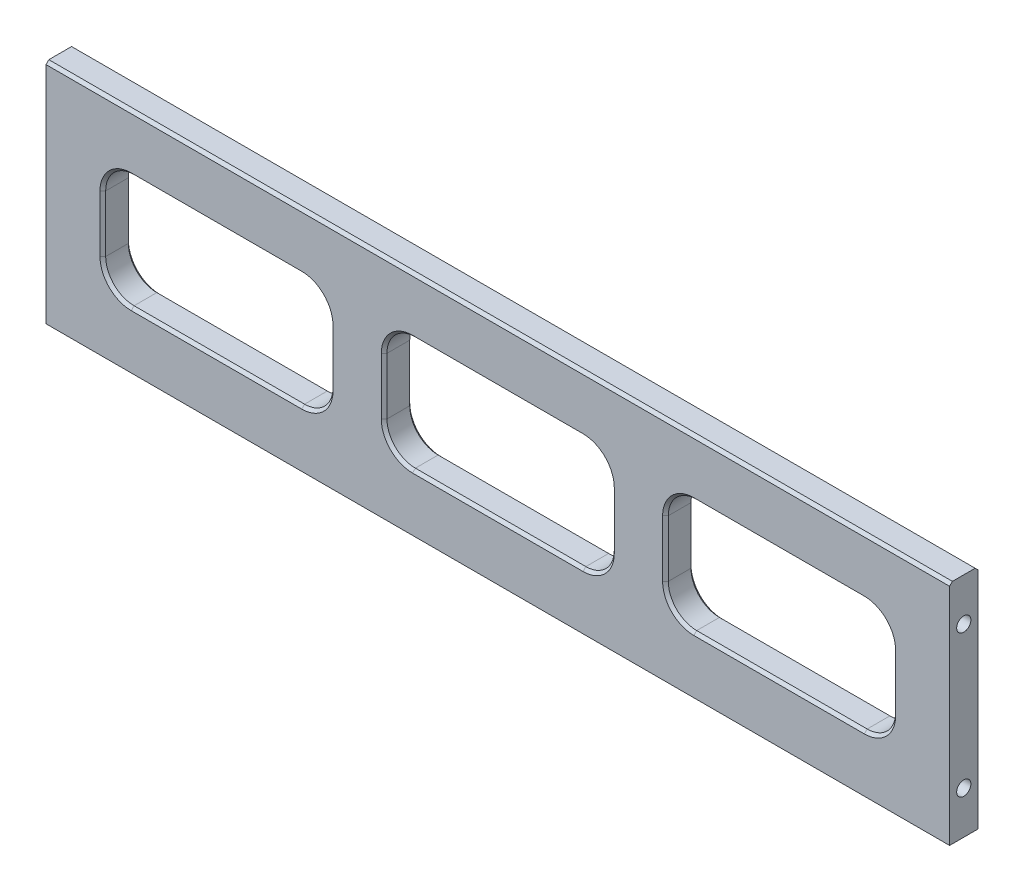
SolidWorks part; units mm, degrees
ref_plane "前视基准面" through (0, 0, 0) normal (0, 0, 1) x (1, 0, 0)
ref_plane "上视基准面" through (0, 0, 0) normal (0, 1, 0) x (1, 0, 0)
ref_plane "右视基准面" through (0, 0, 0) normal (1, 0, 0) x (0, 0, -1)
ref_plane "基准面4" through (0, 0, 10) normal (0, 0, 1) x (1, 0, 0)
sketch "草图1" plane through (0, 0, 10) normal (0, 0, 1) x (1, 0, 0)
  line L0 (-159, -20) -> (-159, -100)
  line L1 (-159, -100) -> (159, -100)
  line L2 (159, -100) -> (159, -20)
  line L3 (159, -20) -> (-159, -20)
extrude "凸台-拉伸1" add sketch "草图1" against normal blind 10
sketch "草图2" plane through (0, 0, 10) normal (0, 0, 1) x (1, 0, 0)
  line L0 (40, -80) -> (40, -40)
  line L1 (40, -40) -> (-40, -40)
  line L2 (-40, -40) -> (-40, -80)
  line L3 (-40, -80) -> (40, -80)
extrude "切除-拉伸1" cut sketch "草图2" against normal through all
sketch "草图3" plane through (0, 0, 10) normal (0, 0, 1) x (1, 0, 0)
  line L0 (139, -80) -> (139, -40)
  line L1 (139, -40) -> (59, -40)
  line L2 (59, -40) -> (59, -80)
  line L3 (59, -80) -> (139, -80)
extrude "切除-拉伸2" cut sketch "草图3" against normal through all
sketch "草图4" plane through (0, 0, 0) normal (0, 0, -1) x (-1, 0, 0)
  line L0 (59, -40) -> (59, -80)
  line L1 (59, -80) -> (139, -80)
  line L2 (139, -80) -> (139, -40)
  line L3 (139, -40) -> (59, -40)
extrude "切除-拉伸3" cut sketch "草图4" against normal through all
hole_wizard "Ø5.0 (5) 直径孔1" positions "草图6" profile "草图5" hole size "Ø5.0" standard "ANSI Metric"
sketch "草图6" plane through (-159, 0, 0) normal (-1, 0, 0) x (0, 0, 1)
  point P0 (5, -35)
  point P1 (5, -85)
sketch "草图5" plane through (-159, -35, 5) normal (0, 1, 0) x (0, 0, 1)
  line L0 (0, 0) -> (0, 16.5022)
  line L1 (0, 16.5022) -> (2.5, 15)
  line L2 (2.5, 15) -> (2.5, 0)
  line L5 (2.5, 0) -> (0, 0)
  line L10 (0, 16.5022) -> (-2.5, 15) construction
  line L11 (0, -6.35) -> (0, 107.95) construction
  dimension "孔直径" = 5
  dimension "孔深度" = 15
  dimension "导头角度" = 118
hole_wizard "Ø5.0 (5) 直径孔2" positions "草图8" profile "草图7" hole size "Ø5.0" standard "ANSI Metric"
sketch "草图8" plane through (159, 0, 0) normal (1, 0, 0) x (0, 0, -1)
  point P0 (-5, -35)
  point P1 (-5, -85)
sketch "草图7" plane through (159, -35, 5) normal (0, 1, 0) x (0, 0, -1)
  line L0 (0, 0) -> (0, 16.5022)
  line L1 (0, 16.5022) -> (2.5, 15)
  line L2 (2.5, 15) -> (2.5, 0)
  line L5 (2.5, 0) -> (0, 0)
  line L10 (0, 16.5022) -> (-2.5, 15) construction
  line L11 (0, -6.35) -> (0, 107.95) construction
  dimension "孔直径" = 5
  dimension "孔深度" = 15
  dimension "导头角度" = 118
hole_wizard "Ø5.0 (5) 直径孔3" positions "草图10" profile "草图9" hole size "Ø5.0" standard "ANSI Metric"
sketch "草图10" plane through (0, -100, 0) normal (0, -1, 0) x (-1, 0, 0)
  point P0 (121.5, -5)
  point P1 (40.5, -5)
  point P2 (-40.5, -5)
  point P3 (-121.5, -5)
sketch "草图9" plane through (-121.5, -100, 5) normal (1, 0, 0) x (0, 0, -1)
  line L0 (0, 0) -> (0, 16.5022)
  line L1 (0, 16.5022) -> (2.5, 15)
  line L2 (2.5, 15) -> (2.5, 0)
  line L5 (2.5, 0) -> (0, 0)
  line L10 (0, 16.5022) -> (-2.5, 15) construction
  line L11 (0, -6.35) -> (0, 107.95) construction
  dimension "孔直径" = 5
  dimension "孔深度" = 15
  dimension "导头角度" = 118
fillet "圆角1" radius 10 12 edges at (40, -40, 5) (139, -40, 5) (-40, -80, 5) (139, -80, 5) (-139, -40, 5) (59, -40, 5) (40, -80, 5) (-59, -40, 5) (-40, -40, 5) (-59, -80, 5) (-139, -80, 5) (59, -80, 5)
chamfer "倒角1" distance 1 angle 45 50 edges at (59, -60, 0) (61.9289, -42.9289, 0) (61.9289, -77.0711, 0) (99, -40, 0) (99, -80, 0) (136.0711, -42.9289, 0) (136.0711, -77.0711, 0) (139, -60, 0) (37.0711, -42.9289, 10) (0, -40, 10) (40, -60, 10) (-37.0711, -42.9289, 10) (37.0711, -77.0711, 10) (-40, -60, 10) (0, -80, 10) (-37.0711, -77.0711, 10) (136.0711, -42.9289, 10) (99, -40, 10) (139, -60, 10) (61.9289, -42.9289, 10) (136.0711, -77.0711, 10) (59, -60, 10) (99, -80, 10) (61.9289, -77.0711, 10) (40, -60, 0) (37.0711, -77.0711, 0) (37.0711, -42.9289, 0) (0, -80, 0) (0, -40, 0) (-37.0711, -77.0711, 0) (-37.0711, -42.9289, 0) (-40, -60, 0) (-136.0711, -42.9289, 10) (-99, -40, 10) (-139, -60, 10) (-61.9289, -42.9289, 10) (-136.0711, -77.0711, 10) (-59, -60, 10) (-99, -80, 10) (-61.9289, -77.0711, 10) (0, -20, 0) (0, -20, 10) (-99, -80, 0) (-61.9289, -77.0711, 0) (-136.0711, -77.0711, 0) (-59, -60, 0) (-139, -60, 0) (-61.9289, -42.9289, 0) (-136.0711, -42.9289, 0) (-99, -40, 0)
